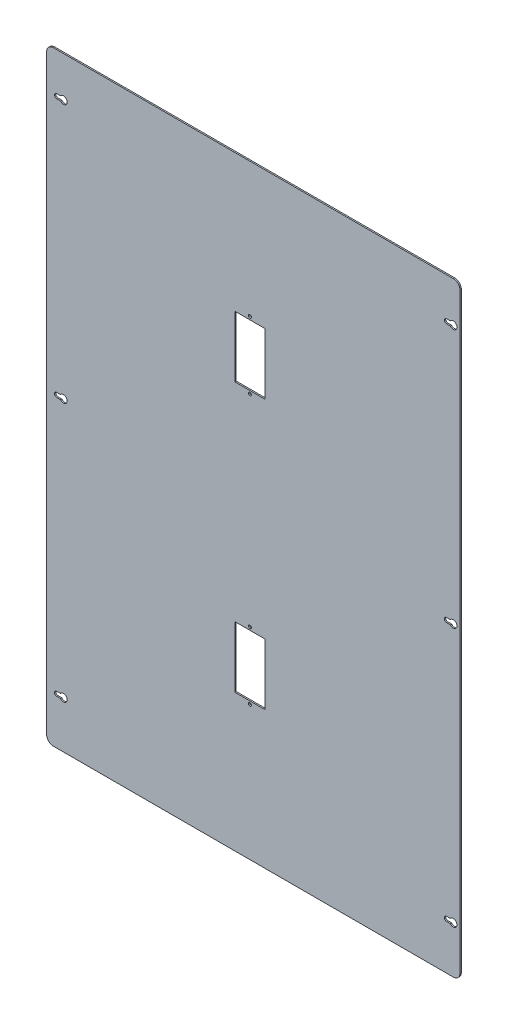
SolidWorks part; units mm, degrees
material "SPCC"
ref_plane "Front Plane" through (0, 0, 0) normal (0, 0, 1) x (1, 0, 0)
ref_plane "Top Plane" through (0, 0, 0) normal (0, 1, 0) x (1, 0, 0)
ref_plane "Right Plane" through (0, 0, 0) normal (1, 0, 0) x (0, 0, -1)
sketch "Sketch1" plane through (0, 0, 0) normal (0, 0, 1) x (1, 0, 0)
  line L1 (-307.5, 450) -> (307.5, 450)
  line L2 (-307.5, 450) -> (-307.5, -450)
  line L3 (-307.5, -450) -> (307.5, -450)
  line L4 (307.5, 450) -> (307.5, -450)
  line L5 (-307.5, 450) -> (307.5, -450) construction
  line L6 (-307.5, -450) -> (307.5, 450) construction
  point P0 (0, 0)
  dimension "D1" = 615
  dimension "D2" = 900
extrude "Boss-Extrude1" add sketch "Sketch1" along normal blind 2
sketch "Sketch7" plane through (0, 0, 0) normal (0, 0, -1) x (-1, 0, 0)
  line L1 (-17.5, 245.5) -> (27.5, 245.5)
  line L2 (-17.5, 245.5) -> (-17.5, 154.5)
  line L3 (-17.5, 154.5) -> (27.5, 154.5)
  line L4 (27.5, 245.5) -> (27.5, 154.5)
  line L5 (-17.5, 245.5) -> (27.5, 154.5) construction
  line L6 (-17.5, 154.5) -> (27.5, 245.5) construction
  line L7 (-17.5, -154.5) -> (27.5, -154.5)
  line L8 (-17.5, -154.5) -> (-17.5, -245.5)
  line L9 (-17.5, -245.5) -> (27.5, -245.5)
  line L10 (27.5, -154.5) -> (27.5, -245.5)
  line L11 (-17.5, -154.5) -> (27.5, -245.5) construction
  line L12 (-17.5, -245.5) -> (27.5, -154.5) construction
  point P0 (5, 200)
  point P5 (5, -200)
  dimension "D1" = 5
  dimension "D2" = 91
  dimension "D3" = 45
  dimension "D4" = 200
  dimension "D5" = 200
extrude "Cut-Extrude4" cut sketch "Sketch7" against normal through all
sketch "Sketch8" plane through (0, 0, 0) normal (0, 0, -1) x (-1, 0, 0)
  line L0 (5, -245.5) -> (5, -154.5) construction
  line L1 (-17.5, -245.5) -> (27.5, -245.5) construction
  line L2 (27.5, -154.5) -> (-17.5, -154.5) construction
  line L3 (-17.5, 154.5) -> (27.5, 154.5) construction
  circle A0 centre (5, 250) radius 2.25
  circle A1 centre (5, 150) radius 2.25
  circle A2 centre (5, -150) radius 2.25
  circle A3 centre (5, -250) radius 2.25
  dimension "D1" = 100
  dimension "D2" = 4.5
  dimension "D3" = 4.5
  dimension "D4" = 100
  dimension "D5" = 4.5
extrude "Cut-Extrude5" cut sketch "Sketch8" against normal through all
fillet "Fillet3" radius 10 4 edges at (307.5, -450, 1) (307.5, 450, 1) (-307.5, 450, 1) (-307.5, -450, 1)
sketch "Sketch10" plane through (0, 0, 0) normal (0, 0, -1) x (-1, 0, 0)
  line L0 (-297.5, 450) -> (297.5, 450) construction
  line L1 (307.5, 440) -> (307.5, -440) construction
  line L2 (292.5, 393.3) -> (286.9, 393.3)
  line L3 (292.5, 386.7) -> (286.9, 386.7)
  arc A0 (292.5, 386.7) -> (292.5, 393.3) centre (292.5, 390) ccw
  arc A1 (286.9, 393.3) -> (286.9, 386.7) centre (282.5, 390) ccw
  dimension "D4" = 11
  dimension "D5" = 6.6
  dimension "D1" = 60
  dimension "D2" = 15
  dimension "D3" = 10
extrude "Cut-Extrude6" cut sketch "Sketch10" against normal blind 10
pattern_linear "LPattern1" count 3 spacing 385 along (0, -1, 0) count 2 spacing 580 along (1, 0, 0) of "Cut-Extrude6"
sketch "Sketch11" plane through (0, 0, 2) normal (0, 0, 1) x (1, 0, 0)
  line L0 (-297.5, -450) -> (297.5, -450) construction
  line L1 (97.5, 560) -> (247.5, 560)
  line L2 (97.5, 560) -> (97.5, 310)
  line L3 (97.5, 310) -> (247.5, 310)
  line L4 (247.5, 560) -> (247.5, 310)
  line L5 (97.5, -140) -> (247.5, -140)
  line L6 (97.5, -140) -> (97.5, -370)
  line L7 (97.5, -370) -> (247.5, -370)
  line L8 (247.5, -140) -> (247.5, -370)
  line L9 (307.5, -440) -> (307.5, 440) construction
  dimension "D1" = 80
  dimension "D2" = 230
  dimension "D3" = 450
  dimension "D4" = 250
  dimension "D5" = 60
  dimension "D6" = 150
extrude "Cut-Extrude7" [suppressed] cut sketch "Sketch11" against normal through all
hole_wizard "M6 Tapped Hole1" positions "Sketch13" profile "Sketch12" tap size "M6" standard "GB"
sketch "Sketch13" plane through (0, 0, 0) normal (0, 0, -1) x (-1, 0, 0)
  point P1 (244.8, -252.75)
  point P4 (244.8, -212.75)
  point P7 (166.1, -194)
  point P10 (166.1, -157.5)
sketch "Sketch12" plane through (-244.8, -252.75, 0) normal (1, 0, 0) x (0, 1, 0)
  line L0 (0, 0) -> (0, 2)
  line L1 (0, 2) -> (2.5, 2)
  line L2 (2.5, 2) -> (2.5, 0)
  line L5 (2.5, 0) -> (0, 0)
  line L11 (0, -6.35) -> (0, 107.95) construction
  dimension "通孔螺纹孔钻头直径" = 5
  dimension "通孔螺纹孔钻头深度" = 2
cosmetic thread "Cosmetic Thread5" [suppressed] parameters "D2"=6
cosmetic thread "Cosmetic Thread6" [suppressed] parameters "D2"=6
cosmetic thread "Cosmetic Thread7" [suppressed] parameters "D2"=6
cosmetic thread "Cosmetic Thread8" [suppressed] parameters "D2"=6
sketch "Sketch14" plane through (0, 0, 0) normal (0, 0, -1) x (-1, 0, 0)
  line L0 (199, -325) -> (199, -370) construction
  line L1 (214, -325) -> (214, -370)
  line L2 (184, -325) -> (184, -370)
  line L3 (307.5, 440) -> (307.5, -440) construction
  line L6 (297.5, -450) -> (-297.5, -450) construction
  circle A1 centre (199, -128.8) radius 17.5
  arc A2 (214, -325) -> (184, -325) centre (199, -325) ccw
  arc A3 (184, -370) -> (214, -370) centre (199, -370) ccw
  point P8 (199, -347.5)
  dimension "D1" = 35
  dimension "D4" = 80
  dimension "D5" = 30
  dimension "D2" = 45
  dimension "D3" = 108.5
sketch "Sketch15" plane through (0, 0, 0) normal (0, 0, -1) x (-1, 0, 0)
  line L2 (-307.5, 350) -> (-227.5, 350) construction
  line L3 (-307.5, -440) -> (-307.5, 440) construction
  line L4 (-307.5, 375) -> (-227.5, 375)
  line L5 (-307.5, 325) -> (-227.5, 325)
  line L6 (-297.5, 450) -> (297.5, 450) construction
  arc A0 (-307.5, 375) -> (-307.5, 325) centre (-307.5, 350) ccw
  arc A1 (-227.5, 325) -> (-227.5, 375) centre (-227.5, 350) ccw
  point P4 (-267.5, 350)
  dimension "D1" = 50
  dimension "D2" = 100
  dimension "D3" = 80
